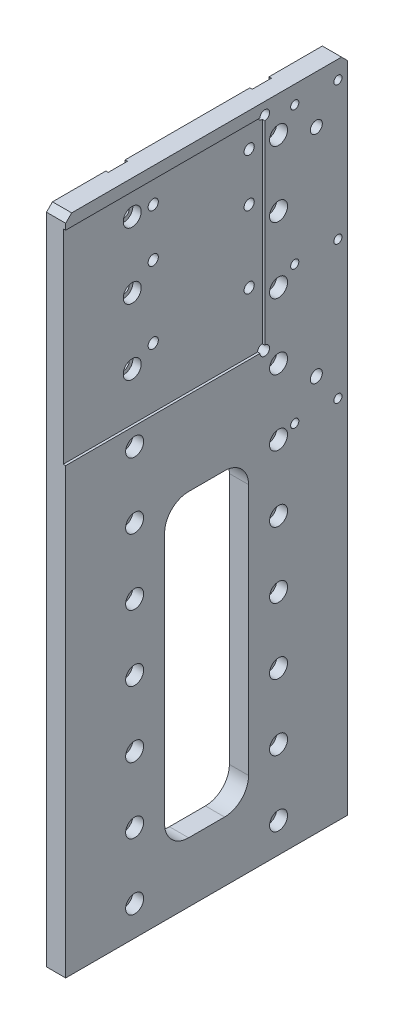
SolidWorks part; units mm, degrees
material "6061-T4 (SS)"
ref_plane "前视基准面" through (0, 0, 0) normal (0, 0, 1) x (1, 0, 0)
ref_plane "上视基准面" through (0, 0, 0) normal (0, 1, 0) x (1, 0, 0)
ref_plane "右视基准面" through (0, 0, 0) normal (1, 0, 0) x (0, 0, -1)
sketch "草图1" plane through (0, 0, 0) normal (0, 0, 1) x (1, 0, 0)
  line L1 (-8, -275) -> (8, -275)
  line L2 (-8, -275) -> (-8, 275)
  line L3 (-8, 275) -> (8, 275)
  line L4 (8, -275) -> (8, 275)
  line L5 (0, 275) -> (0, -275) construction
  line L6 (-8, 0) -> (8, 0) construction
  point P0 (0, 0)
  dimension "D1" = 16
  dimension "D2" = 550
extrude "凸台-拉伸1" add sketch "草图1" along normal blind 235
sketch "草图4" plane through (-8, 0, 0) normal (-1, 0, 0) x (0, 0, 1)
  line L0 (117.5, 275) -> (117.5, -275) construction
  line L3 (235, 275) -> (0, 275) construction
  line L4 (235, -275) -> (0, -275) construction
  line L5 (57.5, 275) -> (57.5, -275) construction
  line L6 (177.5, 275) -> (177.5, -275) construction
  line L8 (49.5, -275) -> (65.5, -275)
  line L9 (49.5, -275) -> (49.5, 275)
  line L10 (49.5, 275) -> (65.5, 275)
  line L11 (65.5, -275) -> (65.5, 275)
  line L12 (57.5, 275) -> (57.5, -275) construction
  line L13 (49.5, 0) -> (65.5, 0) construction
  line L14 (169.5, -275) -> (185.5, -275)
  line L15 (169.5, -275) -> (169.5, 275)
  line L16 (169.5, 275) -> (185.5, 275)
  line L17 (185.5, -275) -> (185.5, 275)
  line L18 (177.5, 275) -> (177.5, -275) construction
  line L19 (169.5, 0) -> (185.5, 0) construction
  point P10 (177.5, 0)
  point P11 (57.5, 0)
  dimension "D1" = 120
  dimension "D2" = 16
extrude "切除-拉伸3" cut sketch "草图4" against normal blind 2
sketch "草图5" plane through (8, 0, 0) normal (1, 0, 0) x (0, 0, -1)
  line L1 (-235, 265) -> (-69, 265)
  line L2 (-235, 265) -> (-235, 95)
  line L3 (-235, 95) -> (-69, 95)
  line L4 (-69, 265) -> (-69, 95)
  line L7 (-235, 275) -> (0, 275) construction
  line L9 (-235, -275) -> (-235, 275) construction
  dimension "D1" = 10
  dimension "D2" = 170
  dimension "D3" = 166
extrude "切除-拉伸4" cut sketch "草图5" against normal blind 2
hole_wizard "M10 螺纹孔1" positions "草图6" profile "草图7" tap size "M10" standard "GB"
sketch "草图6" plane through (6, 0, 0) normal (1, 0, 0) x (0, 0, -1)
  line L11 (-160, 245) -> (-80, 245) construction
  line L12 (-160, 245) -> (-160, 145) construction
  line L13 (-160, 145) -> (-80, 145) construction
  line L14 (-80, 245) -> (-80, 145) construction
  line L15 (-69, 265) -> (-235, 265) construction
  line L19 (-235, 265) -> (-235, 95) construction
  line L20 (-80, 205) -> (-160, 205) construction
  point P156 (-160, 245)
  point P157 (-80, 145)
  point P226 (-160, 145)
  point P227 (-80, 245)
  point P236 (-80, 205)
  point P242 (-160, 205)
  dimension "D1" = 80
  dimension "D2" = 100
  dimension "D3" = 20
  dimension "D4" = 60
  dimension "D6" = 75
sketch "草图7" plane through (6, 245, 160) normal (0, 1, 0) x (0, 0, -1)
  line L0 (0, 0) -> (0, 30.0537)
  line L1 (0, 30.0537) -> (4.25, 27.5)
  line L2 (4.25, 27.5) -> (4.25, 0)
  line L5 (4.25, 0) -> (0, 0)
  line L10 (0, 30.0537) -> (-4.25, 27.5) construction
  line L11 (0, -6.35) -> (0, 107.95) construction
  dimension "螺纹孔钻头直径" = 8.5
  dimension "螺纹孔钻头深度" = 27.5
  dimension "导头角度" = 118
cosmetic thread "孔螺蚊线20" parameters "D1"=14, "D2"=10
cosmetic thread "孔螺蚊线21" parameters "D1"=14, "D2"=10
cosmetic thread "孔螺蚊线22" parameters "D1"=14, "D2"=10
cosmetic thread "孔螺蚊线23" parameters "D1"=14, "D2"=10
cosmetic thread "孔螺蚊线24" parameters "D1"=14, "D2"=10
cosmetic thread "孔螺蚊线25" parameters "D1"=14, "D2"=10
hole_wizard "M8 螺纹孔1" positions "草图8" profile "草图9" tap size "M8" standard "GB"
sketch "草图8" plane through (0, -275, 0) normal (0, -1, 0) x (-1, 0, 0)
  line L0 (0, 0) -> (0, -235) construction
  line L1 (8, -235) -> (-8, -235) construction
  point P9 (0, -72.5)
  point P11 (0, -27.5)
  point P33 (0, -117.5)
  point P35 (0, -162.5)
  point P37 (0, -207.5)
  dimension "D1" = 27.5
  dimension "D2" = 45
  dimension "D3" = 45
  dimension "D4" = 45
  dimension "D5" = 45
sketch "草图9" plane through (0, -275, 207.5) normal (1, 0, 0) x (0, 0, -1)
  line L0 (0, 0) -> (0, 27.0429)
  line L1 (0, 27.0429) -> (3.4, 25)
  line L2 (3.4, 25) -> (3.4, 0)
  line L5 (3.4, 0) -> (0, 0)
  line L10 (0, 27.0429) -> (-3.4, 25) construction
  line L11 (0, -6.35) -> (0, 107.95) construction
  dimension "螺纹孔钻头直径" = 6.8
  dimension "螺纹孔钻头深度" = 25
  dimension "导头角度" = 118
cosmetic thread "孔螺蚊线7" parameters "D1"=20, "D2"=8
cosmetic thread "孔螺蚊线8" parameters "D1"=20, "D2"=8
cosmetic thread "孔螺蚊线9" parameters "D1"=20, "D2"=8
cosmetic thread "孔螺蚊线10" parameters "D1"=20, "D2"=8
cosmetic thread "孔螺蚊线11" parameters "D1"=20, "D2"=8
sketch "草图15" plane through (-8, 0, 0) normal (-1, 0, 0) x (0, 0, 1)
  line L0 (117.5, 275) -> (117.5, -275) construction
  line L1 (169.5, 275) -> (65.5, 275) construction
  line L2 (169.5, -275) -> (65.5, -275) construction
  line L4 (82.5, -225) -> (152.5, -225)
  line L5 (82.5, -225) -> (82.5, 25)
  line L6 (82.5, 25) -> (152.5, 25)
  line L7 (152.5, -225) -> (152.5, 25)
  line L8 (117.5, 25) -> (117.5, -225) construction
  line L9 (82.5, -100) -> (152.5, -100) construction
  point P6 (117.5, -100)
  dimension "D1" = 70
  dimension "D2" = 250
  dimension "D3" = 250
extrude "切除-拉伸5" cut sketch "草图15" against normal blind 16
fillet "圆角1" radius 20 4 edges at (0, -225, 82.5) (0, -225, 152.5) (0, 25, 152.5) (0, 25, 82.5)
chamfer "倒角1" distance 5 angle 45 2 edges at (0, 275, 0) (0, 275, 235)
hole_wizard "打孔尺寸(%根据)内六角圆柱头螺钉的类型1" positions "草图16" profile "草图17" counterbore size "M8" standard "GB"
sketch "草图16" plane through (8, 0, 0) normal (1, 0, 0) x (0, 0, -1)
  line L0 (-117.5, 275) -> (-117.5, -275) construction
  line L1 (-230, 275) -> (-5, 275) construction
  line L2 (-235, -275) -> (0, -275) construction
  line L3 (-177.5, -307.5) -> (-177.5, 275) construction
  line L4 (-57.5, -307.5) -> (-57.5, 275) construction
  line L5 (-177.5, -250) -> (-57.5, -250) construction
  point P15 (-177.5, -250)
  point P19 (-57.5, -250)
  dimension "D1" = 120
  dimension "D2" = 25
sketch "草图17" plane through (8, -250, 57.5) normal (0, 1, 0) x (0, 0, -1)
  line L0 (0, 0) -> (0, 30.2039)
  line L1 (0, 30.2039) -> (4.5, 27.5)
  line L2 (4.5, 27.5) -> (4.5, 9)
  line L3 (4.5, 9) -> (7.5, 9)
  line L4 (7.5, 9) -> (7.5, 0)
  line L5 (7.5, 0) -> (0, 0)
  line L10 (0, 30.2039) -> (-4.5, 27.5) construction
  line L11 (0, -6.35) -> (0, 107.95) construction
  dimension "孔直径" = 9
  dimension "孔深度" = 27.5
  dimension "柱形沉头孔直径" = 15
  dimension "柱形沉头孔深度" = 9
  dimension "导头角度" = 118
pattern_linear "阵列(线性)1" count 10 spacing 55 along (0, 1, 0) of "打孔尺寸(%根据)内六角圆柱头螺钉的类型1"
hole_wizard "M8 螺纹孔2" positions "草图18" profile "草图19" tap size "M8" standard "GB"
sketch "草图18" plane through (8, 0, 0) normal (1, 0, 0) x (0, 0, -1)
  line L2 (-8, 260) -> (-8, 30) construction
  line L4 (-44, 260) -> (-44, 30) construction
  line L5 (-26, 32.5) -> (-26, 272.5) construction
  line L6 (-8, 145) -> (-44, 145) construction
  line L9 (-8, 30) -> (-44, 30) construction
  line L11 (-8, 260) -> (-44, 260) construction
  line L12 (-230, 275) -> (-5, 275) construction
  point P312 (-8, 145)
  point P314 (-44, 145)
  point P323 (-8, 260)
  point P325 (-44, 260)
  point P327 (-8, 30)
  point P329 (-44, 30)
  dimension "D1" = 36
  dimension "D2" = 15
  dimension "D4" = 8
  dimension "D6" = 230
sketch "草图19" plane through (8, 145, 8) normal (0, 1, 0) x (0, 0, -1)
  line L0 (0, 0) -> (0, 24.2929)
  line L1 (0, 24.2929) -> (3.4, 22.25)
  line L2 (3.4, 22.25) -> (3.4, 0)
  line L5 (3.4, 0) -> (0, 0)
  line L10 (0, 24.2929) -> (-3.4, 22.25) construction
  line L11 (0, -6.35) -> (0, 107.95) construction
  dimension "螺纹孔钻头直径" = 6.8
  dimension "螺纹孔钻头深度" = 22.25
  dimension "导头角度" = 118
cosmetic thread "孔螺蚊线12" parameters "D1"=16, "D2"=8
cosmetic thread "孔螺蚊线13" parameters "D1"=16, "D2"=8
cosmetic thread "孔螺蚊线14" parameters "D1"=16, "D2"=8
cosmetic thread "孔螺蚊线15" parameters "D1"=16, "D2"=8
cosmetic thread "孔螺蚊线26" parameters "D1"=16, "D2"=8
cosmetic thread "孔螺蚊线27" parameters "D1"=16, "D2"=8
sketch "草图20" plane through (8, 0, 0) normal (1, 0, 0) x (0, 0, -1)
  circle A0 centre (-69, 95) radius 4
  circle A1 centre (-69, 265) radius 4
  dimension "D1" = 8
extrude "切除-拉伸6" cut sketch "草图20" against normal through all
hole_wizard "大小mm 暗销孔1" positions "草图21" profile "草图22" hole size "Ø10.0" standard "GB"
sketch "草图21" plane through (8, 0, 0) normal (1, 0, 0) x (0, 0, -1)
  line L0 (-44, 30) -> (-44, 145) construction
  line L1 (-8, 30) -> (-8, 145) construction
  line L2 (-8, 30) -> (-44, 30) construction
  line L3 (-26, 30) -> (-26, 264.5432) construction
  point P15 (-26, 55)
  point P17 (-26, 235)
  dimension "D1" = 25
  dimension "D2" = 180
sketch "草图22" plane through (8, 235, 26) normal (0, 1, 0) x (0, 0, -1)
  line L0 (0, 0) -> (0, 13.0043)
  line L1 (0, 13.0043) -> (5, 10)
  line L2 (5, 10) -> (5, 0)
  line L5 (5, 0) -> (0, 0)
  line L10 (0, 13.0043) -> (-5, 10) construction
  line L11 (0, -6.35) -> (0, 107.95) construction
  dimension "孔直径" = 10
  dimension "孔深度" = 10
  dimension "导头角度" = 118
